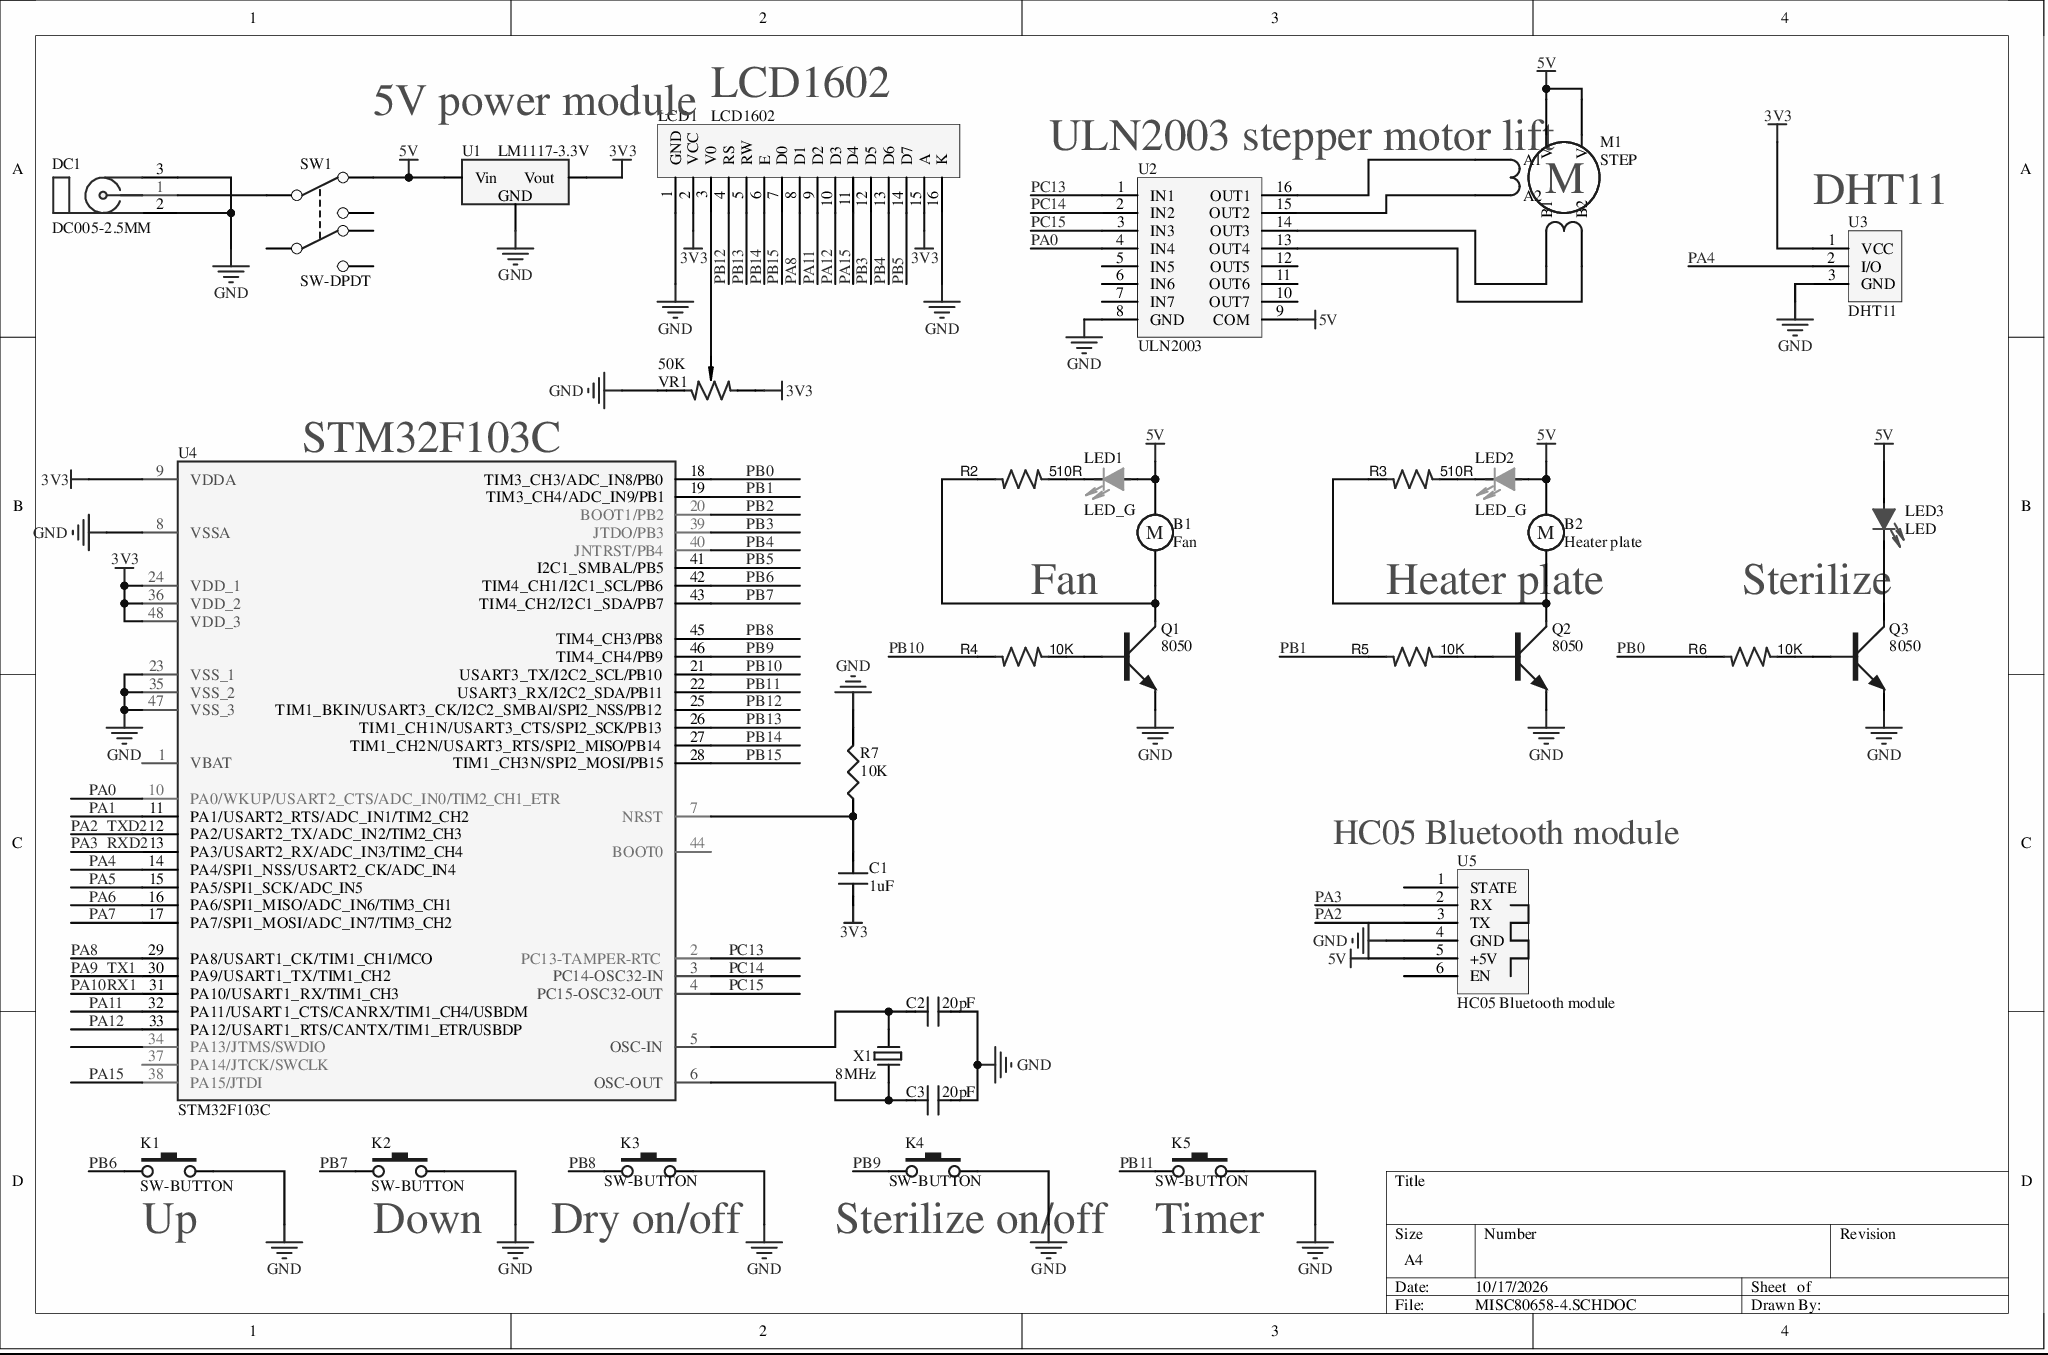
[diagram p0: MISC80658-4.SCHDOC]
# Altium project MISC80658-2.PrjPcb
1 sheet, 33 parts. Net scope: global (net labels, ports and power ports of the same name join across sheets).
Board file: MISC80658.PcbDoc

## Sheet MISC80658-4.SCHDOC
size A4

### Parts
B1  Fan  [RB5-10.5]
B2  Heater plate  [RB5-10.5]
C1  1uF  [C 0805_L]
C2  20pF  [C 0805_L]
C3  20pF  [C 0805_L]
DC1  DC005-2.5MM  [DC-005]
K1  SW-BUTTON  [TSW SMD-3*6*2.5]
K2  SW-BUTTON  [TSW SMD-3*6*2.5]
K3  SW-BUTTON  [TSW SMD-3*6*2.5]
K4  SW-BUTTON  [TSW SMD-3*6*2.5]
K5  SW-BUTTON  [TSW SMD-3*6*2.5]
LCD1  LCD1602  [LCD1602]
LED1  LED_G  [LED 5MM-W]
LED2  LED_G  [LED 5MM-W]
LED3  LED  [LED 5MM-W]
M1  STEP  [DIP-6]
Q1  8050  [SOT-23]
Q2  8050  [SOT-23]
Q3  8050  [SOT-23]
R2  510R  [R 0805_L]
R3  510R  [R 0805_L]
R4  10K  [R 0805_L]
R5  10K  [R 0805_L]
R6  10K  [R 0805_L]
R7  10K  [R 0805_L]
SW1  SW-DPDT  [KFT DIP-7X7]
U1  LM1117-3.3V  [D2PAK]
U2  ULN2003  [DIP16]
U3  DHT11  [HDR1X3]
U4  STM32F103C  [LQFP48 7X7]
U5  HC05 Bluetooth module  [HDR1X6]
VR1  50K  [3296W]
X1  8MHz  [OSC 6035-2P]

### Nets
3V3: C1.1 LCD1.2(VCC) LCD1.15(A) U1.2(Vout) U3.1(VCC) U4.9(VDDA) U4.24(VDD_1) U4.36(VDD_2) U4.48(VDD_3) VR1.1
5V: B1.1 B2.1 LED1.1 LED2.1 LED3.1 M1.4(V) M1.6(V) SW1.2 U1.1(Vin) U2.9(COM) U5.5(+5V)
GND: C2.2 C3.2 DC1.2 DC1.3 K1.2 K2.2 K3.2 K4.2 K5.2 LCD1.1(GND) LCD1.16(K) Q1.E Q2.E Q3.E R7.2 U1.3(GND) U2.8(GND) U3.3(GND) U4.8(VSSA) U4.23(VSS_1) U4.35(VSS_2) U4.47(VSS_3) U5.4(GND) VR1.2
PA0: U2.4(IN4) U4.10(PA0/WKUP/USART2_CTS/ADC_IN0/TIM2_CH1_ETR)
PA1: U4.11(PA1/USART2_RTS/ADC_IN1/TIM2_CH2)
PA2: U4.12(PA2/USART2_TX/ADC_IN2/TIM2_CH3) U5.3(TX)  [also labelled TXD2]
PA3: U4.13(PA3/USART2_RX/ADC_IN3/TIM2_CH4) U5.2(RX)  [also labelled RXD2]
PA4: U3.2(I/O) U4.14(PA4/SPI1_NSS/USART2_CK/ADC_IN4)
PA5: U4.15(PA5/SPI1_SCK/ADC_IN5)
PA6: U4.16(PA6/SPI1_MISO/ADC_IN6/TIM3_CH1)
PA7: U4.17(PA7/SPI1_MOSI/ADC_IN7/TIM3_CH2)
PA8: LCD1.8(D1) U4.29(PA8/USART1_CK/TIM1_CH1/MCO)
PA9: U4.30(PA9/USART1_TX/TIM1_CH2)  [also labelled TX1]
PA10: U4.31(PA10/USART1_RX/TIM1_CH3)  [also labelled RX1]
PA11: LCD1.9(D2) U4.32(PA11/USART1_CTS/CANRX/TIM1_CH4/USBDM)
PA12: LCD1.10(D3) U4.33(PA12/USART1_RTS/CANTX/TIM1_ETR/USBDP)
PA15: LCD1.11(D4) U4.38(PA15/JTDI)
PB0: R6.1 U4.18(TIM3_CH3/ADC_IN8/PB0)
PB1: R5.1 U4.19(TIM3_CH4/ADC_IN9/PB1)
PB2: U4.20(BOOT1/PB2)
PB3: LCD1.12(D5) U4.39(JTDO/PB3)
PB4: LCD1.13(D6) U4.40(JNTRST/PB4)
PB5: LCD1.14(D7) U4.41(I2C1_SMBAL/PB5)
PB6: K1.1 U4.42(TIM4_CH1/I2C1_SCL/PB6)
PB7: K2.1 U4.43(TIM4_CH2/I2C1_SDA/PB7)
PB8: K3.1 U4.45(TIM4_CH3/PB8)
PB9: K4.1 U4.46(TIM4_CH4/PB9)
PB10: R4.1 U4.21(USART3_TX/I2C2_SCL/PB10)
PB11: K5.1 U4.22(USART3_RX/I2C2_SDA/PB11)
PB12: LCD1.4(RS) U4.25(TIM1_BKIN/USART3_CK/I2C2_SMBAl/SPI2_NSS/PB12)
PB13: LCD1.5(RW) U4.26(TIM1_CH1N/USART3_CTS/SPI2_SCK/PB13)
PB14: LCD1.6(E) U4.27(TIM1_CH2N/USART3_RTS/SPI2_MISO/PB14)
PB15: LCD1.7(D0) U4.28(TIM1_CH3N/SPI2_MOSI/PB15)
PC13: U2.1(IN1) U4.2(PC13-TAMPER-RTC)
PC14: U2.2(IN2) U4.3(PC14-OSC32-IN)
PC15: U2.3(IN3) U4.4(PC15-OSC32-OUT)
NetB1_2: B1.2 Q1.C R2.1
NetB2_2: B2.2 Q2.C R3.1
NetC1_2: C1.2 R7.1 U4.7(NRST)
NetC2_1: C2.1 U4.5(OSC-IN) X1.1
NetC3_1: C3.1 U4.6(OSC-OUT) X1.2
NetDC1_1: DC1.1(VCC) SW1.1
NetLCD1_3: LCD1.3(V0) VR1.3(W)
NetLED1_2: LED1.2 R2.2
NetLED2_2: LED2.2 R3.2
NetLED3_2: LED3.2 Q3.C
NetM1_1: M1.1(A1) U2.16(OUT1)
NetM1_3: M1.3(A2) U2.15(OUT2)
NetM1_4: M1.4(B1) U2.14(OUT3)
NetM1_6: M1.6(B2) U2.13(OUT4)
NetQ1_B: Q1.B R4.2
NetQ2_B: Q2.B R5.2
NetQ3_B: Q3.B R6.2

Not connected (* = marked no-connect by the designer): SW1 3 4 5 6; U2 5(IN5) 6(IN6) 7(IN7) 10(OUT7) 11(OUT6) 12(OUT5); U4 1(VBAT) 34(PA13/JTMS/SWDIO) 37(PA14/JTCK/SWCLK) 44(BOOT0); U5 1(STATE) 6(EN)

### Notes on the sheet
- 5V power module
- LCD1602
- (near M1) ULN2003 stepper motor lift
- (near U3) DHT11
- (near U4) STM32F103C
- (near Q1) Fan
- (near B2) Heater plate
- Sterilize
- (near U5) HC05 Bluetooth module
- (near K1) Up
- (near K2) Down
- (near K3) Dry on/off
- Sterilize on/off
- (near K5) Timer

### Library data of the parts
B1 = Motor: 5V fan; Published: 24-Mar-1999; LatestRevisionDate: 17-Jul-2002; LatestRevisionNote: Re-released for DXP Platform.; PackageReference: RB5-10.5; Publisher: COMPANY_A
B2 = Motor: Published: 24-Mar-1999; LatestRevisionDate: 17-Jul-2002; LatestRevisionNote: Re-released for DXP Platform.; PackageReference: RB5-10.5; Publisher: COMPANY_A
C1-C3 = CAP: Chip capacitor
DC1 = DC005-2.5MM: BOM_Manufacturer: SOFNG; BOM_Supplier: LCSC; BOM_Manufacturer Part: DC005-2.5MM; BOM_Supplier Part: C111573; spicePre: D; spiceSymbolName: DC005-2.5MM
K1-K5 = SW-BUTTON: Tact switch
LCD1 = LCD1602: LCD module
LED1 LED2 = LED_G: Green LED
M1 = MOTOR STEPPER-4_-2: Stepper motor
Q1-Q3 = NPN: NPN transistor
R2-R6 = RES: Resistor
R7 = RES1
SW1 = SW-DPDT: DPDT switch
U1 = LM78xx: Voltage regulator circuit
U2 = ULN2003: ULN2003 driver IC
U3 = DS18B20: DHT11 temperature/humidity
U4 = STM32F103C8T6: 48-pin LQFP
U5 = HC-05-蓝牙模块: HC-05 Bluetooth module
VR1 = RW: Potentiometer
X1 = CRYSTAL: Crystal oscillator